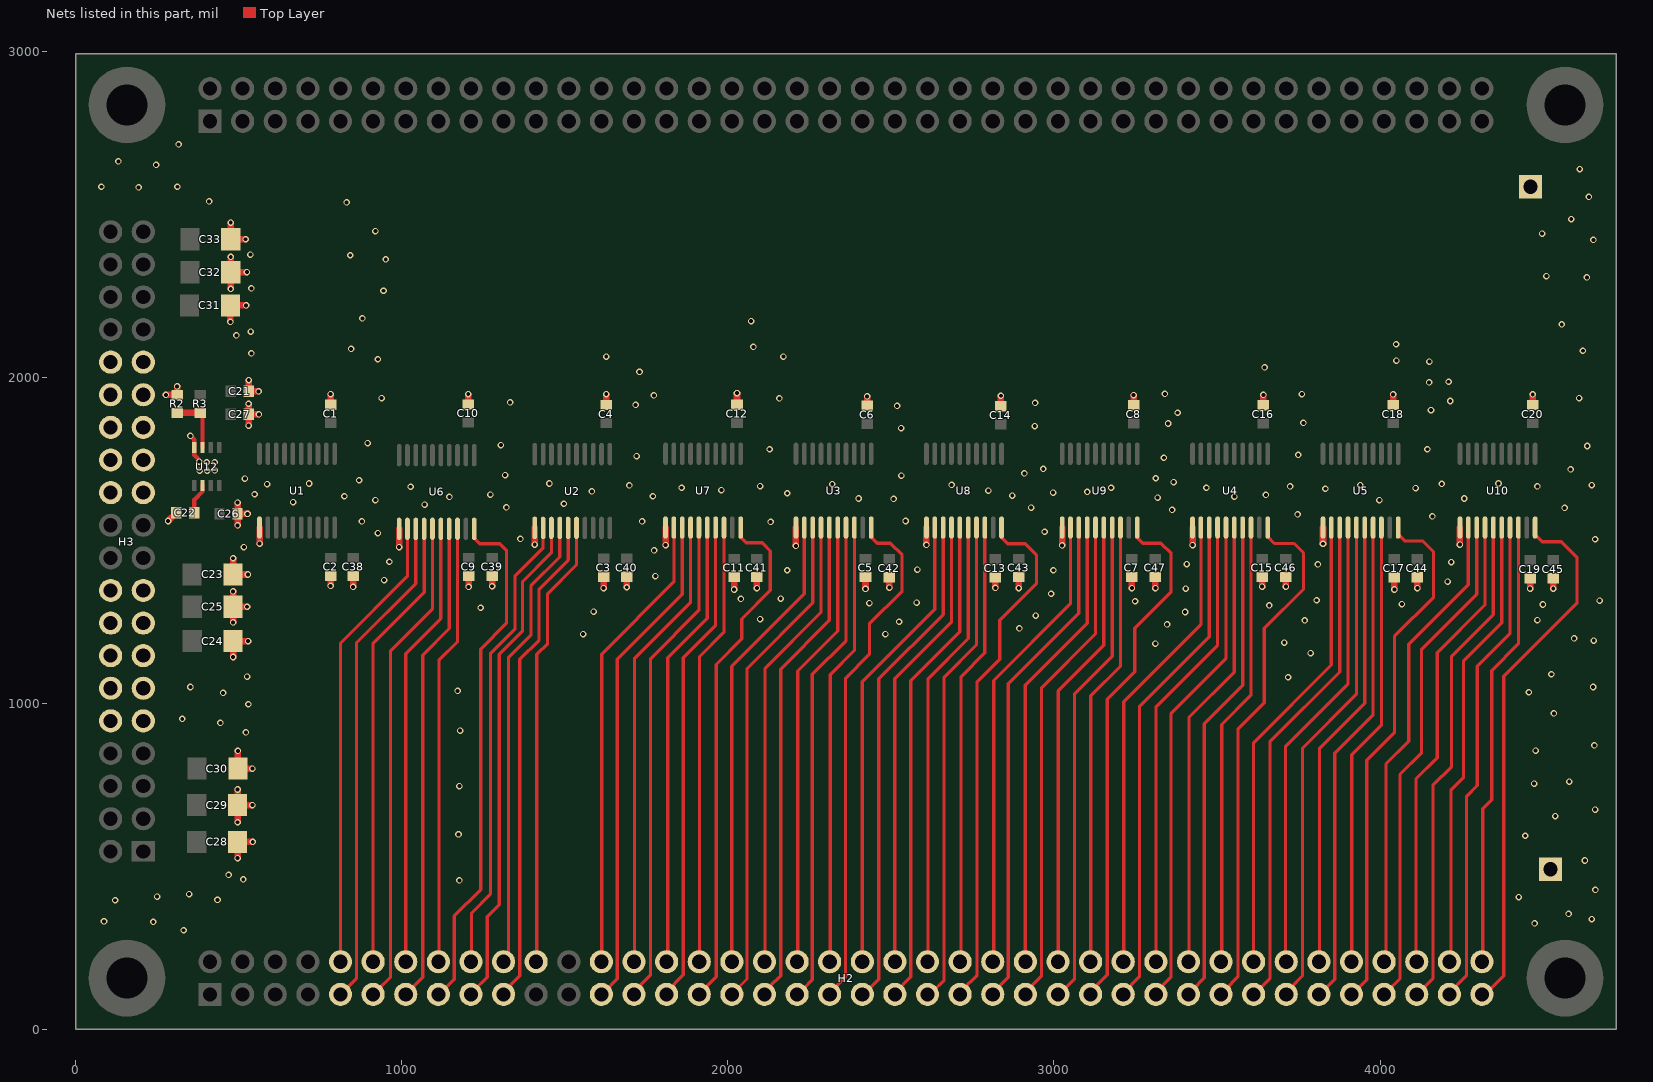
[diagram p0: the nets of this part, all layers, seen from the top]
# Altium PCB MISC79033.pcbdoc (part 2 of 2)
Units mil, origin at the board's own origin, x right, y up, seen from the top; angles counter-clockwise.
Board outline 4724.41 x 2992.13 mil, 4 copper layers (Top Layer, GND, POWER, Bottom Layer); 59 components, 166 nets, 504 pads, 319 vias.

## Via types
v1: diameter 20, hole 12, Top Layer to Bottom Layer, 319 vias

## Nets (pads, with @x,y where several pads share a name; then routed paths per layer and width w, separated by ;. In a path a pad name is that pad's centre, name@x,y a point inside that pad or via, vN(x,y) a via of type N, cw(c..) or ccw(c..) an arc to the next point about the centre after c; other vN are vias at no path point) (continued)
B24: H2.22 U2.16 | length 1406.4
  Top Layer w10: H2.22@1414,223 1414,296 ; 1414,255 1414,296 ; U2.16@1535.8,1537.97 1535.8,1424.8 1447,1336 1447,1183 1414,1150 1414,296
B25: H2.19 U2.15 | length 1493.8
  Top Layer w10: H2.19@1320,123 1362,165 1362,1135 1421,1194 1421,1350 1510.2,1439.2 U2.15@1510.2,1537.97
B26: H2.20 U2.14 | length 1431.3
  Top Layer w10: H2.20@1327,210 1327,295 ; 1327,257 1327,295 ; U2.14@1484.61,1537.97 1484.61,1448.61 1396,1360 1396,1209 1327,1140 1327,295
B27: H2.17 U2.13 | length 1514.7
  Top Layer w10: H2.17@1223,121 1262,160 1262,346 1299,383 1299,1150 1370,1221 1370,1372 1459.02,1461.02 U2.13@1459.02,1537.97
B28: H2.18 U2.12 | length 1484.9
  Top Layer w10: H2.18@1214,223 1214,338 ; 1214,259 1214,338 ; U2.12@1433.43,1537.97 1433.43,1476.43 1347,1390 1347,1227 1272,1152 1272,415 1214,357 1214,338
B31: H2.39 U3.20 | length 1556.6
  Top Layer w10: H2.39@2329,130 2361,162 2361,1077 2434,1150 2434,1244 2534,1344 2534,1455 2498,1491 2458,1491 2439.16,1509.84 U3.20@2439.16,1538.97
B32: H2.40 U3.18 | length 1384.4
  Top Layer w10: H2.40@2312,210 2314,212 2314,281 ; 2314,257 2314,281 ; U3.18@2387.98,1538.97 2387.98,1161.98 2314,1088 2314,281
B33: H2.37 U3.17 | length 1465.1
  Top Layer w10: H2.37@2234,127 2259,152 2259,267 2259,1089 2362.39,1192.39 U3.17@2362.39,1538.97
B34: H2.38 U3.16 | length 1404.9
  Top Layer w10: H2.38@2214,222 2214,291 ; 2214,253.91 2214,291 ; U3.16@2336.8,1538.97 2336.8,1221.8 2214,1099 2214,291
B35: H2.35 U3.15 | length 1482.4
  Top Layer w10: H2.35@2129,132 2162,165 2162,1105 2311.2,1254.2 U3.15@2311.2,1538.97
B36: H2.36 U3.14 | length 1416.1
  Top Layer w10: H2.36@2114,221 2114,284 ; 2114,257 2114,284 ; U3.14@2285.61,1538.97 2285.61,1278.61 2114,1107 2114,284
B37: H2.33 U3.13 | length 1506.8
  Top Layer w10: H2.33@2031,127 2058.64,154.64 2058.64,1106.64 2260.02,1308.02 U3.13@2260.02,1538.97
B38: H2.34 U3.12 | length 1407.1
  Top Layer w10: H2.34@2012,224 2012,1113 2234.43,1335.43 U3.12@2234.43,1538.97
B41: H2.63 U4.20 | length 1595.6
  Top Layer w10: H2.63@3526,123 3564,161 3564,921 3645,1002 3645,1230 3765,1350 3765,1461 3736,1490 3676,1490 3655.16,1510.84 U4.20@3655.16,1538.97
B42: H2.64 U4.18 | length 1372.2
  Top Layer w10: H2.64@3514,222 3514,281 ; 3514,263 3514,281 ; U4.18@3603.98,1538.97 3603.98,1024.98 3514,935 3514,281
B43: H2.61 U4.17 | length 1480.5
  Top Layer w10: H2.61@3425,122 3461,158 3461,164 3461,938 3578.39,1055.39 U4.17@3578.39,1538.97
B44: H2.62 U4.16 | length 1383.5
  Top Layer w10: H2.62@3414,237 3414,278 ; 3414,253.91 3414,278 ; U4.16@3552.8,1538.97 3552.8,1095.8 3414,957 3414,278
B45: H2.59 U4.15 | length 1512.7
  Top Layer w10: H2.59@3313,115 3359,161 3359,969 3527.2,1137.2 U4.15@3527.2,1538.97
B46: H2.60 U4.14 | length 1414.1
  Top Layer w10: H2.60@3313,226 3313,281 ; 3313,258 3313,281 ; U4.14@3501.61,1538.97 3501.61,1178.61 3313,990 3313,281
B47: H2.57 U4.13 | length 1537.3
  Top Layer w10: H2.57@3212,111 3262,161 3262,990 3476.02,1204.02 U4.13@3476.02,1538.97
B48: H2.58 U4.12 | length 1436.9
  Top Layer w10: H2.58@3214,226 3214,283 ; 3214,257 3214,283 ; U4.12@3450.43,1538.97 3450.43,1241.43 3214,1005 3214,283
B51: H2.71 U5.20 | length 1601.5
  Top Layer w10: H2.71@3922,115 3959,152 3959,825 4044,910 4044,1205 4164,1325 4164,1464 4130,1498 4075,1498 4055.16,1517.84 U5.20@4055.16,1538.97
B52: H2.72 U5.18 | length 1381.7
  Top Layer w10: H2.72@3913,225 3913,294 ; 3913,264 3913,294 ; U5.18@4003.98,1538.97 4003.98,932.98 3913,842 3913,294
B53: H2.69 U5.17 | length 1468.9
  Top Layer w10: H2.69@3836,129 3861,154 3861,847 3978.39,964.39 U5.17@3978.39,1538.97
B54: H2.70 U5.16 | length 1389.5
  Top Layer w10: H2.70@3814,221 3814,271 ; 3814,257 3814,271 ; U5.16@3952.8,1538.97 3952.8,999.8 3814,861 3814,271
B55: H2.67 U5.15 | length 1491.9
  Top Layer w10: H2.67@3727,130 3762,165 3762,862 3927.2,1027.2 U5.15@3927.2,1538.97
B56: H2.68 U5.14 | length 1412.3
  Top Layer w10: H2.68@3710,228 3710,281 ; 3710,259 3710,281 ; U5.14@3901.61,1538.97 3901.61,1060.61 3710,869 3710,281
B57: H2.65 U5.13 | length 1523.9
  Top Layer w10: H2.65@3625,119 3662,156 3662,882 3876.02,1096.02 U5.13@3876.02,1538.97
B58: H2.66 U5.12 | length 1444.6
  Top Layer w10: H2.66@3610,221 3612,223 3612,283 ; 3612,256 3612,283 ; U5.12@3850.43,1538.97 3850.43,1117.43 3612,879 3612,283
B61: H2.15 U6.20 | length 1574
  Top Layer w10: H2.15@1126,119 1161,154 1161,348 1242,429 1242,1166 1321,1245 1321,1469 1301,1489 1239,1489 1222.16,1505.84 U6.20@1222.16,1534.97
B62: H2.16 U6.18 | length 1338.6
  Top Layer w10: H2.16@1114,220 1114,1132 1170.98,1188.98 1170.98,1231.02 1170.98,1238 U6.18@1170.98,1534.97
B63: H2.13 U6.17 | length 1466
  Top Layer w10: H2.13@1027,123 1064,160 1064,1148 1145.39,1229.39 1145.39,1258 ; 1145.39,1253 1145.39,1258 ; U6.17@1145.39,1534.97 1145.39,1258
B64: H2.14 U6.16 | length 1365.8
  Top Layer w10: H2.14@1012,234 1012,1152 1119.8,1259.8 U6.16@1119.8,1534.97 ; H2.14@1013,224 H2.14@1013,234 ; H2.14@1017.5,224 1017.5,214.5 H2.14@1018,214
B65: H2.11 U6.15 | length 1483.6
  Top Layer w10: H2.11@926,121 965.77,160.77 965.77,1160.77 1094,1289 1094,1328 ; 1094.2,1328 U6.15@1094.2,1534.97
B66: H2.12 U6.14 | length 1365.8
  Top Layer w10: H2.12@912,234 912,1184 1068.61,1340.61 U6.14@1068.61,1534.97
B67: H2.9 U6.13 | length 1512.3
  Top Layer w10: H2.9@820,115 861,156 861,1185 1043.02,1367.02 U6.13@1043.02,1534.97
B68: H2.10 U6.12 | length 1412.5
  Top Layer w10: H2.10@812.2,207.48 812.2,1184.2 1017.43,1389.43 U6.12@1017.43,1534.97
B71: H2.31 U7.20 | length 1568.6
  Top Layer w10: H2.31@1924,122 1964,162 1964,1119 2042.5,1197.5 2042.5,1258.5 2130,1346 2130,1467 2105,1492 2056,1492 2039.16,1508.84 U7.20@2039.16,1538.97
B72: H2.32 U7.18 | length 1371
  Top Layer w10: H2.32@1913,226 1913,281 ; 1913,254 1913,281 ; U7.18@1987.98,1538.97 1987.98,1217.98 1913,1143 1913,281
B73: H2.29 U7.17 | length 1485.3
  Top Layer w10: H2.29@1812,116 1863,167 1863,1140 1962.39,1239.39 U7.17@1962.39,1538.97
B74: H2.30 U7.16 | length 1386.1
  Top Layer w10: H2.30@1816,224 1816,275 ; 1816,253.91 1816,275 ; U7.16@1936.8,1538.97 1936.8,1260.8 1816,1140 1816,275
B75: H2.27 U7.15 | length 1497
  Top Layer w10: H2.27@1718,122 1763,167 1763,1137 1911.2,1285.2 U7.15@1911.2,1538.97
B76: H2.28 U7.14 | length 1379.1
  Top Layer w10: H2.28@1714,231 1714,1138 1885.61,1309.61 U7.14@1885.61,1538.97
B77: H2.25 U7.13 | length 1521.6
  Top Layer w10: H2.25@1622,116 1661,155 1661,161 1661,1135 1860.02,1334.02 U7.13@1860.02,1538.97
B78: H2.26 U7.12 | length 1448.7
  Top Layer w10: H2.26@1613,205 1613,281 ; 1613,258 1613,281 ; U7.12@1834.43,1538.97 1834.43,1372.43 1613,1151 1613,281
B81: H2.47 U8.20 | length 1587.9
  Top Layer w10: H2.47@2719,121 2764,166 2764,1066 2833.5,1135.5 2833.5,1254.5 2946,1367 2946,1455 2912,1489 2858,1489 2839.16,1507.84 U8.20@2839.16,1538.97
B82: H2.48 U8.18 | length 1391.3
  Top Layer w10: H2.48@2710,226 2715,231 2715,303 ; 2715,257 2715,303 ; U8.18@2787.98,1538.97 2787.98,1154.98 2715,1082 2715,303
B83: H2.45 U8.17 | length 1477.2
  Top Layer w10: H2.45@2629,117 2663,151 2663,158 2663,1080 2762.39,1179.39 U8.17@2762.39,1538.97
B84: H2.46 U8.16 | length 1413.7
  Top Layer w10: H2.46@2612,209 2614,211 2614,287 ; 2614,255 2614,287 ; U8.16@2736.8,1538.97 2736.8,1198.8 2614,1076 2614,287
B85: H2.43 U8.15 | length 1506.7
  Top Layer w10: H2.43@2514,114 2561,161 2561,1069 2711.2,1219.2 U8.15@2711.2,1538.97
B86: H2.44 U8.14 | length 1383.9
  Top Layer w10: H2.44@2512,227 2512,1075 2685.61,1248.61 U8.14@2685.61,1538.97
B87: H2.41 U8.13 | length 1518.9
  Top Layer w10: H2.41@2426,117 2463,154 2463,162 2463,1075 2660.02,1272.02 U8.13@2660.02,1538.97
B88: H2.42 U8.12 | length 1429.1
  Top Layer w10: H2.42@2412,223 2412,282 ; 2412,261 2412,282 ; U8.12@2634.43,1538.97 2634.43,1288.43 2412,1066 2412,282
B91: H2.55 U9.20 | length 1597.3
  Top Layer w10: H2.55@3114,119 3163,168 3163,1012 3247.5,1096.5 3247.5,1230.5 3359,1342 3359,1460 3328,1491 3272,1491 3255.16,1507.84 U9.20@3255.16,1538.97
B92: H2.56 U9.18 | length 1400.7
  Top Layer w10: H2.56@3113,221 3113,299 ; 3113,253.91 3113,299 ; U9.18@3203.98,1538.97 3203.98,1113.98 3113,1023 3113,299
B93: H2.53 U9.17 | length 1491.2
  Top Layer w10: H2.53@3021,113 3063,155 3063,1029 3178.39,1144.39 U9.17@3178.39,1538.97
B94: H2.54 U9.16 | length 1437
  Top Layer w10: H2.54@3013,222 3013,316 ; 3013,253.91 3013,316 ; U9.16@3152.8,1538.97 3152.8,1177.8 3013,1038 3013,316
B95: H2.51 U9.15 | length 1516.9
  Top Layer w10: H2.51@2910,112 2962,164 2962,1048 3127.2,1213.2 U9.15@3127.2,1538.97
B96: H2.52 U9.14 | length 1430.6
  Top Layer w10: H2.52@2912,221 2912,288 ; 2912,253.91 2912,288 ; U9.14@3101.61,1538.97 3101.61,1245.61 2912,1056 2912,288
B97: H2.49 U9.13 | length 1537.7
  Top Layer w10: H2.49@2811,111 2860,160 2860,1060 3076.02,1276.02 U9.13@3076.02,1538.97
B98: H2.50 U9.12 | length 1484.5
  Top Layer w10: H2.50@2815,215 2815,343 ; 2815,280 2815,343 ; U9.12@3050.43,1538.97 3050.43,1305.43 2815,1070 2815,343
B101: H2.79 U10.20 | length 1626.8
  Top Layer w10: H2.79@4329,114 4379,164 4379,1083 4604,1308 4604,1447 4556,1495 4497,1495 4475.16,1516.84 U10.20@4475.16,1538.97
B102: H2.80 U10.18 | length 1399.1
  Top Layer w10: H2.80@4315,213 4315,292 ; 4315,264 4315,292 ; U10.18@4423.98,1538.97 4423.98,1181.98 4342,1100 4342,704 4315,677 4315,292
B103: H2.77 U10.17 | length 1494.7
  Top Layer w10: H2.77@4218,119 4265,166 4265,715 4298,748 4298,1114 4398.39,1214.39 U10.17@4398.39,1538.97
B104: H2.78 U10.16 | length 1433.5
  Top Layer w10: H2.78@4217,213 4217,303 ; 4217,260 4217,303 ; U10.16@4372.8,1538.97 4372.8,1246.8 4256,1130 4256,773 4217,734 4217,303
B105: H2.75 U10.15 | length 1513.4
  Top Layer w10: H2.75@4124,118 4162,156 4162,749 4219,806 4219,1144 4347.2,1272.2 U10.15@4347.2,1538.97
B106: H2.76 U10.14 | length 1410.6
  Top Layer w10: H2.76@4110,216 4110,768 4175,833 4175,1155 4321.61,1301.61 U10.14@4321.61,1538.97
B107: H2.73 U10.13 | length 1535.5
  Top Layer w10: H2.73@4022,117 4061,156 4061,782 4127,848 4127,1166 4296.02,1335.02 U10.13@4296.02,1538.97
B108: H2.74 U10.12 | length 1531.5
  Top Layer w10: H2.74@4018,229 4018,373 ; 4018,256 4018,373 ; U10.12@4270.43,1538.97 4270.43,1363.43 4088,1181 4088,884 4018,814 4018,373
GND: C1.1 C2.1 C3.1 C4.1 C5.1 C6.1 C7.1 C8.1 C9.1 C10.1 C11.1 C12.1 C13.1 C14.1 C15.1 C16.1 C17.1 C18.1 C19.1 C20.1 C21.1 C22.1 C23.1 C24.1 C25.1 C26.2 C27.1 C28.1 C29.1 C30.1 C31.1 C32.1 C33.1 C38.1 C39.1 C40.1 C41.1 C42.1 C43.1 C44.1 C45.1 C46.1 C47.1 H3.9 H3.10 H3.11 H3.12 H3.13 H3.14 H3.15 H3.16 H3.17 H3.18 H3.23 H3.24 H3.25 H3.26 H3.27 H3.28 H3.29 H3.30 H3.31 H3.32 pad.1 R2.1 U1.11 U2.11 U3.11 U4.11 U5.11 U6.11 U7.11 U8.11 U9.11 U10.11 U12.4 | length 2966.2
  Top Layer w13: v1(352,1820) 363.6,1808.4 U12.4@363.6,1784.1 363.6,1761.4 373,1752
  Top Layer w20: v1(276.56,1945.55) R2.1@311,1945.55 v1(311,1972) ; v1(283.44,1559) C22.1@308.44,1584 ; v1(474.58,2169.42) C31.1@474.58,2220 v1(523,2220) ; v1(475.7,2270.7) C32.1@475.7,2322 ; v1(475.7,2368.7) C32.1@475.7,2322 ; v1(475.7,2473.7) C33.1@475.7,2423 v1(521,2423) ; v1(482.7,1444.7) C23.1@482.7,1395 v1(528,1395) ; v1(483.02,1142.02) C24.1@483.02,1191 v1(529,1191) ; v1(483.02,1247.98) C25.1@483.02,1296 ; v1(483.02,1343.02) C25.1@483.02,1296 ; v1(496.56,1545.44) C26.2@496.56,1581 ; v1(496.56,1615.44) C26.2@496.56,1581 ; v1(496.7,525.3) C28.1@496.7,575 v1(543,575) ; v1(496.7,635.3) C29.1@496.7,688 ; v1(496.7,735.7) C29.1@496.7,688 ; v1(497.7,854.3) C30.1@497.7,800 v1(542,800) ; v1(525,2322) C32.1@475.7,2322 ; v1(526,1296) C25.1@483.02,1296 ; v1(527,1581) C26.2@496.56,1581 ; v1(530.56,1851.44) C27.1@530.56,1886 ; v1(530.56,1918.55) C27.1@530.56,1886 ; v1(530.81,1990.81) C21.1@530.81,1956.22 v1(561.22,1956.22) ; v1(542,688) C29.1@496.7,688 ; v1(562,1886) C27.1@530.56,1886 ; v1(563.84,1489.84) U1.11@563.84,1538.97 ; v1(782,1360) C2.1@782,1390.44 ; C1.1@782,1915.55 v1(782,1948) ; v1(851,1357) C38.1@851,1390.44 ; v1(991.84,1479.16) U6.11@991.84,1534.97 ; C10.1@1204,1916.55 v1(1204,1948) ; v1(1205,1357) C9.1@1205,1390.44 ; v1(1277,1359) C39.1@1277,1390.44 ; v1(1407.84,1486.84) U2.11@1407.84,1537.97 ; v1(1619,1353) C3.1@1619,1388.44 ; C4.1@1627,1914.55 v1(1627,1948) ; v1(1690,1356) C40.1@1690,1388.44 ; v1(1808.84,1484.84) U7.11@1808.84,1538.97 ; v1(2019,1349) C11.1@2019,1387.44 ; C12.1@2028,1915.55 v1(2028,1951) ; v1(2089,1353) C41.1@2089,1387.44 ; v1(2208.84,1482.84) U3.11@2208.84,1538.97 ; v1(2422,1351) C5.1@2422,1387.44 ; C6.1@2427,1912.55 v1(2427,1941) ; v1(2495,1355) C42.1@2495,1386.44 ; v1(2608.84,1485.84) U8.11@2608.84,1538.97 ; v1(2820,1354) C13.1@2820,1386.44 ; C14.1@2837,1910.55 v1(2837,1943) ; v1(2892,1353) C43.1@2892,1387.44 ; v1(3024.84,1484.16) U9.11@3024.84,1538.97 ; v1(3239,1353) C7.1@3239,1387.44 ; C8.1@3244,1913.55 v1(3244,1945) ; v1(3311,1353) C47.1@3311,1387.44 ; v1(3424.84,1484.84) U4.11@3424.84,1538.97 ; v1(3638,1358) C15.1@3638,1387.44 ; C16.1@3642,1913.55 v1(3642,1946) ; v1(3711,1358) C46.1@3711,1387.44 ; v1(3824.84,1489.16) U5.11@3824.84,1538.97 ; C18.1@4040,1914.55 v1(4040,1947) ; v1(4044,1349) C17.1@4044,1386.44 ; v1(4114,1353) C44.1@4114,1386.44 ; v1(4244.84,1486.84) U10.11@4244.84,1538.97 ; v1(4460,1352) C19.1@4460,1383.44 ; C20.1@4468,1914.55 v1(4468,1947) ; v1(4531,1352) C45.1@4531,1383.44
  other v1: 331,304 4474,325 238,330 87,331 4649,338 4578,354 121,396 435,397 4425,406 250,407 348,415 4660,428 1177,457 514,460 469,474 4628,518 4445,594 1174,598 4537,654 4659,674 1177,746 4472,754 4580,760 4477,855 4657,871 522,911 1179,916 444,940 327,952 4533,969 530,997 452,1032 4456,1034 1171,1038 352,1050 4653,1050 3718,1080 526,1082 4525,1089 3787,1154 3311,1183 3706,1186 4655,1192 4595,1199 1556,1212 2483,1212 2894,1230 3347,1242 2525,1250 3769,1254 4482,1255 2099,1258 2944,1269 3402,1280 1588,1281 1242,1293 3660,1300 4499,1303 4067,1304 2434,1307 2579,1309 3249,1313 4673,1315 3805,1316 2040,1320 2162,1321 2991,1336 3404,1352 4207,1373 946,1378 1778,1390 2182,1408 2998,1408 2581,1410 3809,1426 3407,1427 4218,1433 962,1434 1774,1469 516,1479 4659,1503 1364,1504 927,1522 2971,1526 2131,1556 878,1558 1737,1558 2545,1559 4160,1573 3747,1579 3362,1593 4566,1599 2930,1600 1321,1601 1070,1609 1497,1612 667,1617 919,1623 3998,1623 2508,1627 2401,1628 4258,1628 3318,1631 1146,1633 3553,1634 824,1635 1770,1635 2872,1637 3650,1639 1272,1640 549,1641 2182,1644 2997,1646 3102,1648 1583,1650 2799,1652 1980,1654 3832,1658 4109,1660 1858,1661 3175,1661 3467,1661 1027,1664 3724,1665 4482,1665 2099,1666 1698,1668 3939,1669 4649,1669 2686,1670 587,1672 2320,1672 4189,1673 716,1674 1453,1674 4363,1674 3367,1678 869,1684 519,1689 3312,1690 2532,1698 1317,1700 2909,1705 380,1713 403,1713 426,1714 4584,1717 2967,1719 402,1739 426,1739 379,1741 3337,1753 1720,1758 3749,1762 2128,1779 4145,1779 4635,1789 1304,1792 895,1798 2531,1844 2941,1850 3350,1858 3765,1860 3379,1891 4156,1899 2519,1912 1717,1915 2942,1921 1332,1923 4215,1927 2158,1935 938,1936 4610,1936 1773,1944 3760,1948 3340,1949 4150,1984 4210,1986 1729,2016 3646,2030 4151,2048 4050,2051 927,2055 1627,2063 2170,2063 539,2073 4622,2081 845,2087 2078,2093 4049,2101 493,2128 537,2140 4557,2162 2071,2172 879,2180 944,2265 539,2272 4634,2306 4510,2310 951,2361 842,2374 536,2376 4654,2421 4497,2440 919,2448 4586,2485 831,2536 409,2539 4640,2553 193,2582 79,2584 312,2584 4612,2638 247,2651 131,2662 316,2714
NetC22_2: C22.2 U12.6 | length 81.3
  Top Layer w13: C22.2@364,1597 364,1624 389.2,1649.2 U12.6@389.2,1667.9
NetR2_2: R2.2 R3.2 U12.3 | length 157.7
  Top Layer w13: U12.3@389.2,1784.1 R3.2@389.2,1879.2
  Top Layer w20: R2.2@311,1890.44 R3.2@373.56,1890.44

## Polygon pours and split planes (outlines as drawn)
GND on Top Layer "Bottom Layer-No Net" (solid, remove dead copper): -296,2926 -296,-177 -143,-330 -95,-378 300,-378 4740,-378 4958,-160 5047,-71 5047,-7 5047,2950 4845,3152 4813,3184 4805,3184 -143,3184 -264,3063 -296,3031 -296,2934
1.8V on Top Layer "Bottom Layer-No Net" (solid, remove dead copper): 362,1966 362,1934 364,1932 367,1929 379,1929 405,1929 408,1926 416,1918 416,1910 416,1864 412,1860 408,1856 408,1803 408,1771 410,1769 411,1768 419,1768 483,1768 493,1778 498,1783 498,1789 498,2048 409,2137 390,2156 390,2220 390,2473 374,2489 365,2498 350,2498 75,2498 69,2492 57,2480 57,2439 57,2132 66,2123 77,2112 104,2112 270,2112 271,2111 279,2103 279,2072 279,2049 362,1966
+5V on Top Layer "Bottom Layer-No Net" (solid, remove dead copper): 64,1543 64,1525 64,1430 84,1410 112,1410 239,1410 252,1397 260,1389 260,1346 260,1160 275,1145 283,1137 321,1137 380,1137 391,1148 393,1150 393,1178 393,1436 409,1452 458,1501 458,1567 458,1679 454,1683 451,1686 447,1686 410,1686 408,1684 405,1681 405,1674 405,1643 397,1635 393,1631 393,1618 393,1555 386,1548 378,1540 343,1540 269,1540 264,1545 261,1548 261,1560 261,1569 250,1580 243,1587 223,1587 82,1587 68,1573 64,1569 64,1543
3.3V on Top Layer "Bottom Layer-No Net" (solid, remove dead copper, pour order 1000): 67,839 67,821 67,518 77,508 94,491 199,491 386,491 394,499 401,506 401,527 401,855 386,870 373,883 215,883 89,883 75,869 67,861 67,839
GND on Bottom Layer "Bottom Layer-No Net" (solid, remove dead copper): -252,2942 -252,-106 -135,-223 -93,-265 141,-265 4804,-265 4942,-127 4984,-85 4984,-32 4984,3059 4878,3165 4750,3293 4623,3293 -135,3293 -273,3155 -273,2985
GND on GND (split plane): 4704.31,20.1 20.1,20.1 20.1,2972.03 4704.31,2972.03
3.3V on POWER (split plane): 4704.31,20.1 20.1,20.1 20.1,1454.91 607,1454.91 609.61,1455.26 612.04,1456.26 614.13,1457.87 799.18,1642.91 4704.31,1642.91
1.8V on POWER (split plane): 4704.31,1663.09 795,1663.09 792.39,1662.74 791.68,1662.45 789.96,1661.73 787.87,1660.13 602.82,1475.09 20.1,1475.09 20.1,2972.03 4704.31,2972.03

## Keep-outs
Keep-Out Layer:
  the board outline again, w10

## Other copper
POWER (plane layer: these items are gaps in the copper):
  lines w20: 15,1465 607,1465 795,1653 4716,1653

## Silkscreen, mask and mechanical layers (free items; w line width, h text height)
Top Overlay:
  text "A37" at 1979,2697 h40
  text "A31" at 2284,2697 h40
  text "A87" at 2379,2697 h40
  text "A81" at 2684,2697 h40
  text "A27" at 1183,2696 h40
  text "A21" at 1488,2696 h40
  text "A77" at 1578,2696 h40
  text "A71" at 1883,2696 h40
  text "A33" at 2184,2696 h40
  text "A83" at 2584,2696 h40
  text "A97" at 2782,2696 h40
  text "A91" at 3087,2696 h40
  text "A47" at 3182,2696 h40
  text "A41" at 3487,2696 h40
  text "A17" at 379,2695 h40
  text "A11" at 684,2695 h40
  text "A67" at 783,2695 h40
  text "A61" at 1088,2695 h40
  text "A23" at 1388,2695 h40
  text "A73" at 1783,2695 h40
  text "A35" at 2082,2695 h40
  text "A85" at 2482,2695 h40
  text "A93" at 2987,2695 h40
  text "A43" at 3387,2695 h40
  text "A13" at 584,2694 h40
  text "A63" at 988,2694 h40
  text "A25" at 1286,2694 h40
  text "A75" at 1681,2694 h40
  text "A95" at 2885,2694 h40
  text "A45" at 3285,2694 h40
  text "A15" at 482,2693 h40
  text "A65" at 886,2693 h40
  text "A57" at 3579,2693 h40
  text "A51" at 3884,2693 h40
  text "A53" at 3784,2692 h40
  text "A55" at 3682,2691 h40
  text "A107" at 3978,2691 h40
  text "A101" at 4283,2691 h40
  text "A103" at 4183,2690 h40
  text "A105" at 4081,2689 h40
  text "A38" at 1977,2652 h40
  text "A32" at 2282,2652 h40
  text "A88" at 2377,2652 h40
  text "A82" at 2682,2652 h40
  text "A28" at 1181,2651 h40
  text "A22" at 1486,2651 h40
  text "A78" at 1576,2651 h40
  text "A72" at 1881,2651 h40
  text "A34" at 2182,2651 h40
  text "A84" at 2582,2651 h40
  text "A98" at 2780,2651 h40
  text "A92" at 3085,2651 h40
  text "A48" at 3180,2651 h40
  text "A42" at 3485,2651 h40
  text "A18" at 377,2650 h40
  text "A12" at 682,2650 h40
  text "A68" at 781,2650 h40
  text "A62" at 1086,2650 h40
  text "A24" at 1386,2650 h40
  text "A74" at 1781,2650 h40
  text "A94" at 2985,2650 h40
  text "A44" at 3385,2650 h40
  text "A14" at 582,2649 h40
  text "A64" at 986,2649 h40
  text "A36" at 2078,2649 h40
  text "A86" at 2478,2649 h40
  text "A16" at 480,2648 h40
  text "A26" at 1282,2648 h40
  text "A76" at 1677,2648 h40
  text "A96" at 2881,2648 h40
  text "A46" at 3281,2648 h40
  text "A58" at 3577,2648 h40
  text "A52" at 3882,2648 h40
  text "A66" at 882,2647 h40
  text "A54" at 3782,2647 h40
  text "A108" at 3976,2646 h40
  text "A102" at 4281,2646 h40
  text "A56" at 3678,2645 h40
  text "A104" at 4181,2645 h40
  text "A106" at 4077,2643 h40
  text "GND" at 4424,2481 h40
  text "1.8V" at 43,2413 h40 r90
  text "1.8V" at 42,2310 h40 r90
  text "1.8V" at 42,2208 h40 r90
  text "1.8V" at 42,2109 h40 r90
  text "GND" at 44,2006 h40 r90
  text "GND" at 44,1905 h40 r90
  text "GND" at 43,1803 h40 r90
  text "GND" at 44,1699 h40 r90
  text "GND" at 43,1603 h40 r90
  text "5V" at 43,1528 h40 r90
  text "5V" at 44,1427 h40 r90
  text "GND" at 43,1308 h40 r90
  text "GND" at 42,1210 h40 r90
  text "GND" at 41,1105 h40 r90
  text "GND" at 42,1009 h40 r90
  text "GND" at 42,906 h40 r90
  text "3.3V" at 42,804 h40 r90
  text "3.3V" at 42,708 h40 r90
  text "3.3V" at 43,613 h40 r90
  text "GND" at 4487,561 h40
  text "3.3V" at 42,512 h40 r90
  text "B108" at 3984,350 h40
  text "B102" at 4289,350 h40
  text "B98" at 2788,349 h40
  text "B92" at 3093,349 h40
  text "B58" at 3583,349 h40
  text "B52" at 3888,349 h40
  text "B10" at 4189,349 h40
  text "B88" at 2386,348 h40
  text "B82" at 2691,348 h40
  text "B94" at 2993,348 h40
  text "B54" at 3788,348 h40
  text "B84" at 2591,347 h40
  text "B106" at 4085,347 h40
  text "B96" at 2889,346 h40
  text "B48" at 3191,346 h40
  text "B42" at 3496,346 h40
  text "B56" at 3684,346 h40
  text "B86" at 2487,345 h40
  text "B44" at 3396,345 h40
  text "B38" at 1988,343 h40
  text "B32" at 2293,343 h40
  text "B46" at 3292,343 h40
  text "B34" at 2193,342 h40
  text "B78" at 1585,340 h40
  text "B72" at 1890,340 h40
  text "B36" at 2089,340 h40
  text "B28" at 1189,339 h40
  text "B22" at 1494,339 h40
  text "B74" at 1790,339 h40
  text "B24" at 1394,338 h40
  text "B76" at 1686,337 h40
  text "B26" at 1290,336 h40
  text "B68" at 790,332 h40
  text "B62" at 1095,332 h40
  text "B64" at 995,331 h40
  text "B18" at 389,329 h40
  text "B12" at 694,329 h40
  text "B66" at 891,329 h40
  text "B14" at 594,328 h40
  text "B16" at 490,326 h40
  text "B107" at 3984,301 h40
  text "B101" at 4289,301 h40
  text "B97" at 2788,300 h40
  text "B91" at 3093,300 h40
  text "B57" at 3583,300 h40
  text "B51" at 3888,300 h40
  text "B103" at 4189,300 h40
  text "B87" at 2386,299 h40
  text "B81" at 2691,299 h40
  text "B93" at 2993,299 h40
  text "B53" at 3788,299 h40
  text "B105" at 4087,299 h40
  text "B83" at 2591,298 h40
  text "B95" at 2891,298 h40
  text "B55" at 3686,298 h40
  text "B85" at 2489,297 h40
  text "B47" at 3191,297 h40
  text "B41" at 3496,297 h40
  text "B43" at 3396,296 h40
  text "B45" at 3294,295 h40
  text "B37" at 1988,294 h40
  text "B31" at 2293,294 h40
  text "B33" at 2193,293 h40
  text "B35" at 2091,292 h40
  text "B77" at 1585,291 h40
  text "B71" at 1890,291 h40
  text "B27" at 1189,290 h40
  text "B21" at 1494,290 h40
  text "B73" at 1790,290 h40
  text "B23" at 1394,289 h40
  text "B75" at 1688,289 h40
  text "B25" at 1292,288 h40
  text "B67" at 790,283 h40
  text "B61" at 1095,283 h40
  text "B63" at 995,282 h40
  text "B65" at 893,281 h40
  text "B17" at 389,280 h40
  text "B11" at 694,280 h40
  text "B13" at 594,279 h40
  text "B15" at 492,278 h40